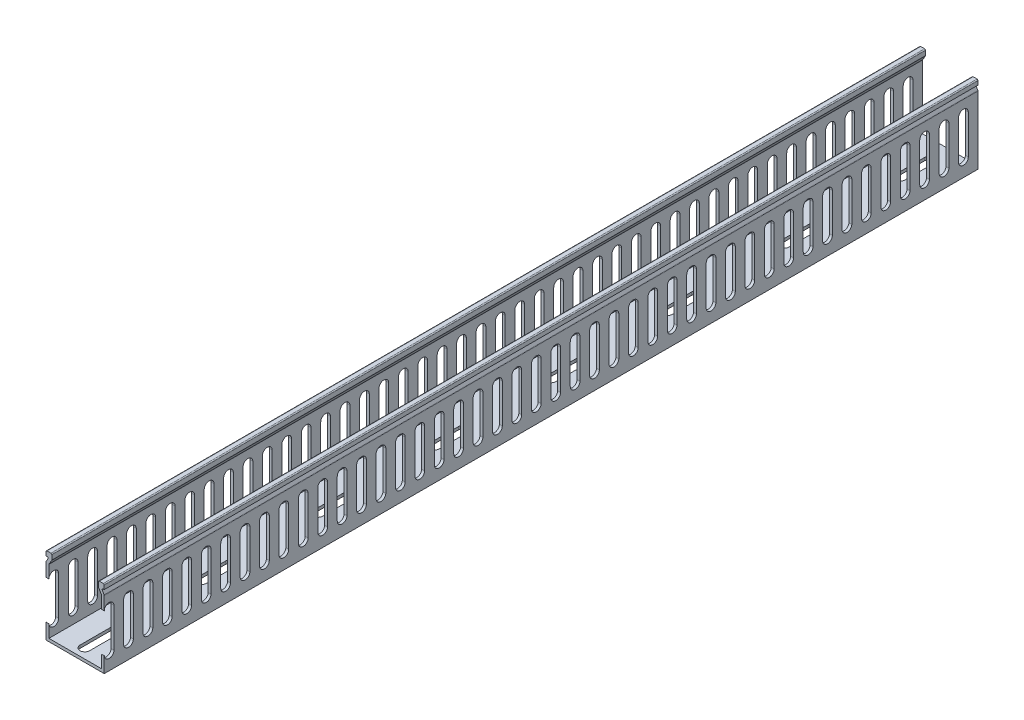
SolidWorks part; units mm, degrees
ref_plane "前基準面" through (0, 0, 0) normal (0, 0, 1) x (1, 0, 0)
ref_plane "上基準面" through (0, 0, 0) normal (0, 1, 0) x (1, 0, 0)
ref_plane "右基準面" through (0, 0, 0) normal (1, 0, 0) x (0, 0, -1)
sketch "草圖1" plane through (0, 0, 0) normal (0, 0, 1) x (1, 0, 0)
  line L0 (0, 0) -> (0, 65.5929) construction
  line L1 (14.9287, 35.1188) -> (13.9543, 36.7428)
  line L2 (14.3831, 37.5) -> (15, 37.5)
  line L3 (15, 37.5) -> (15, 39.5)
  line L4 (-15, 0) -> (15, 0)
  line L5 (15, 34.8615) -> (15, 0)
  line L6 (14.5, 40) -> (12.5, 40)
  line L7 (12, 39.5) -> (12, 37.223)
  line L8 (12.0713, 36.9658) -> (13.4287, 34.7033)
  line L9 (13.5, 34.446) -> (13.5, 1.5)
  line L10 (13.5, 1.5) -> (-13.5, 1.5)
  line L11 (-13.5, 34.446) -> (-13.5, 1.5)
  line L12 (-12.0713, 36.9658) -> (-13.4287, 34.7033)
  line L13 (-12, 39.5) -> (-12, 37.223)
  line L14 (-14.5, 40) -> (-12.5, 40)
  line L15 (-15, 34.8615) -> (-15, 0)
  line L16 (-15, 37.5) -> (-15, 39.5)
  line L17 (-14.3831, 37.5) -> (-15, 37.5)
  line L18 (-14.9287, 35.1188) -> (-13.9543, 36.7428)
  arc A0 (13.9543, 36.7428) -> (14.3831, 37.5) centre (14.3831, 37) cw
  arc A1 (14.5, 40) -> (15, 39.5) centre (14.5, 39.5) cw
  arc A2 (12, 39.5) -> (12.5, 40) centre (12.5, 39.5) cw
  arc A3 (12.0713, 36.9658) -> (12, 37.223) centre (12.5, 37.223) cw
  arc A4 (13.5, 34.446) -> (13.4287, 34.7033) centre (13, 34.446) ccw
  arc A5 (15, 34.8615) -> (14.9287, 35.1188) centre (14.5, 34.8615) ccw
  arc A6 (-15, 34.8615) -> (-14.9287, 35.1188) centre (-14.5, 34.8615) cw
  arc A7 (-13.5, 34.446) -> (-13.4287, 34.7033) centre (-13, 34.446) cw
  arc A8 (-12.0713, 36.9658) -> (-12, 37.223) centre (-12.5, 37.223) ccw
  arc A9 (-12, 39.5) -> (-12.5, 40) centre (-12.5, 39.5) ccw
  arc A10 (-14.5, 40) -> (-15, 39.5) centre (-14.5, 39.5) ccw
  arc A11 (-13.9543, 36.7428) -> (-14.3831, 37.5) centre (-14.3831, 37) ccw
  point P15 (13.5, 37.5)
  point P18 (15, 40)
  point P27 (15, 35)
  point P47 (0, 1.5)
  point P49 (-15, 35)
  point P50 (-15, 40)
  point P51 (-13.5, 37.5)
  dimension "D2" = 1.5
  dimension "D3" = 1.5
  dimension "D10" = 0.5
  dimension "D4" = 35
  dimension "D5" = 1.5
  dimension "D1" = 15
  dimension "D6" = 3
  dimension "D7" = 2.5
  dimension "D8" = 2.5
  dimension "D9" = 1.5
extrude "伸長1" add sketch "草圖1" along normal blind 450
sketch "草圖2" plane through (-15, 0, 0) normal (-1, 0, 0) x (0, 0, 1)
  line L0 (0, 34.8615) -> (0, 0) construction
  line L2 (5, 28) -> (5, 8)
  line L4 (10, 28) -> (10, 8)
  arc A0 (10, 28) -> (5, 28) centre (7.5, 28) ccw
  arc A1 (5, 8) -> (10, 8) centre (7.5, 8) ccw
  dimension "D1" = 5
  dimension "D2" = 20
  dimension "D3" = 5
extrude "伸長2" cut sketch "草圖2" against normal through all
pattern_linear "直線複製排列1" count 130 spacing 10 along (0, 0, 1) of "伸長2"
sketch "草圖3" plane through (0, 0, 0) normal (0, -1, 0) x (1, 0, 0)
  line L2 (-2.5, 25) -> (-2.5, 10)
  line L4 (2.5, 25) -> (2.5, 10)
  arc A0 (2.5, 25) -> (-2.5, 25) centre (0, 25) ccw
  arc A1 (-2.5, 10) -> (2.5, 10) centre (0, 10) ccw
  dimension "D2" = 5
  dimension "D1" = 15
  dimension "D4" = 2.5
extrude "伸長3" cut sketch "草圖3" against normal through all
pattern_linear "直線複製排列2" count 25 spacing 60 along (0, 0, 1) of "伸長3"
